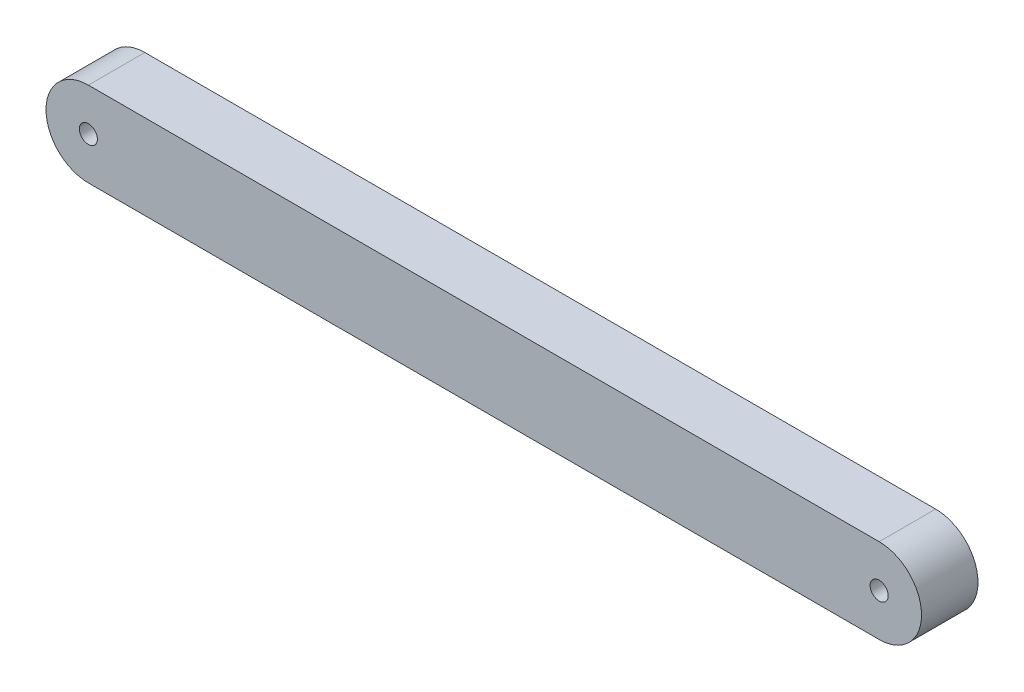
from build123d import *

# Parameters (mm, degrees)
EXTRUDE_1_DEPTH     = 10
SKETCH_2_R          = 3.2
CUT_EXTRUDE_1_DEPTH = 25


with BuildPart() as part:
    # 草图1 → 凸台-拉伸1 (new, symmetric)
    with BuildSketch(Plane.XY):
        with BuildLine():
            Line((-140, 15), (140, 15))
            ThreePointArc((140, 15), (155, 0), (140, -15))
            Line((140, -15), (-140, -15))
            ThreePointArc((-140, -15), (-155, 0), (-140, 15))
        make_face()
    extrude(amount=EXTRUDE_1_DEPTH, both=True)

    # 草图2 → 切除-拉伸1 (cut, symmetric)
    with BuildSketch(Plane.XY):
        with Locations(Location((-140, 0, 0), (0, 0, 180))):
            Circle(SKETCH_2_R)
        with Locations(Location((140, 0, 0), (0, 0, 180))):
            Circle(SKETCH_2_R)
    extrude(amount=CUT_EXTRUDE_1_DEPTH, both=True, mode=Mode.SUBTRACT)


solid = part.part
